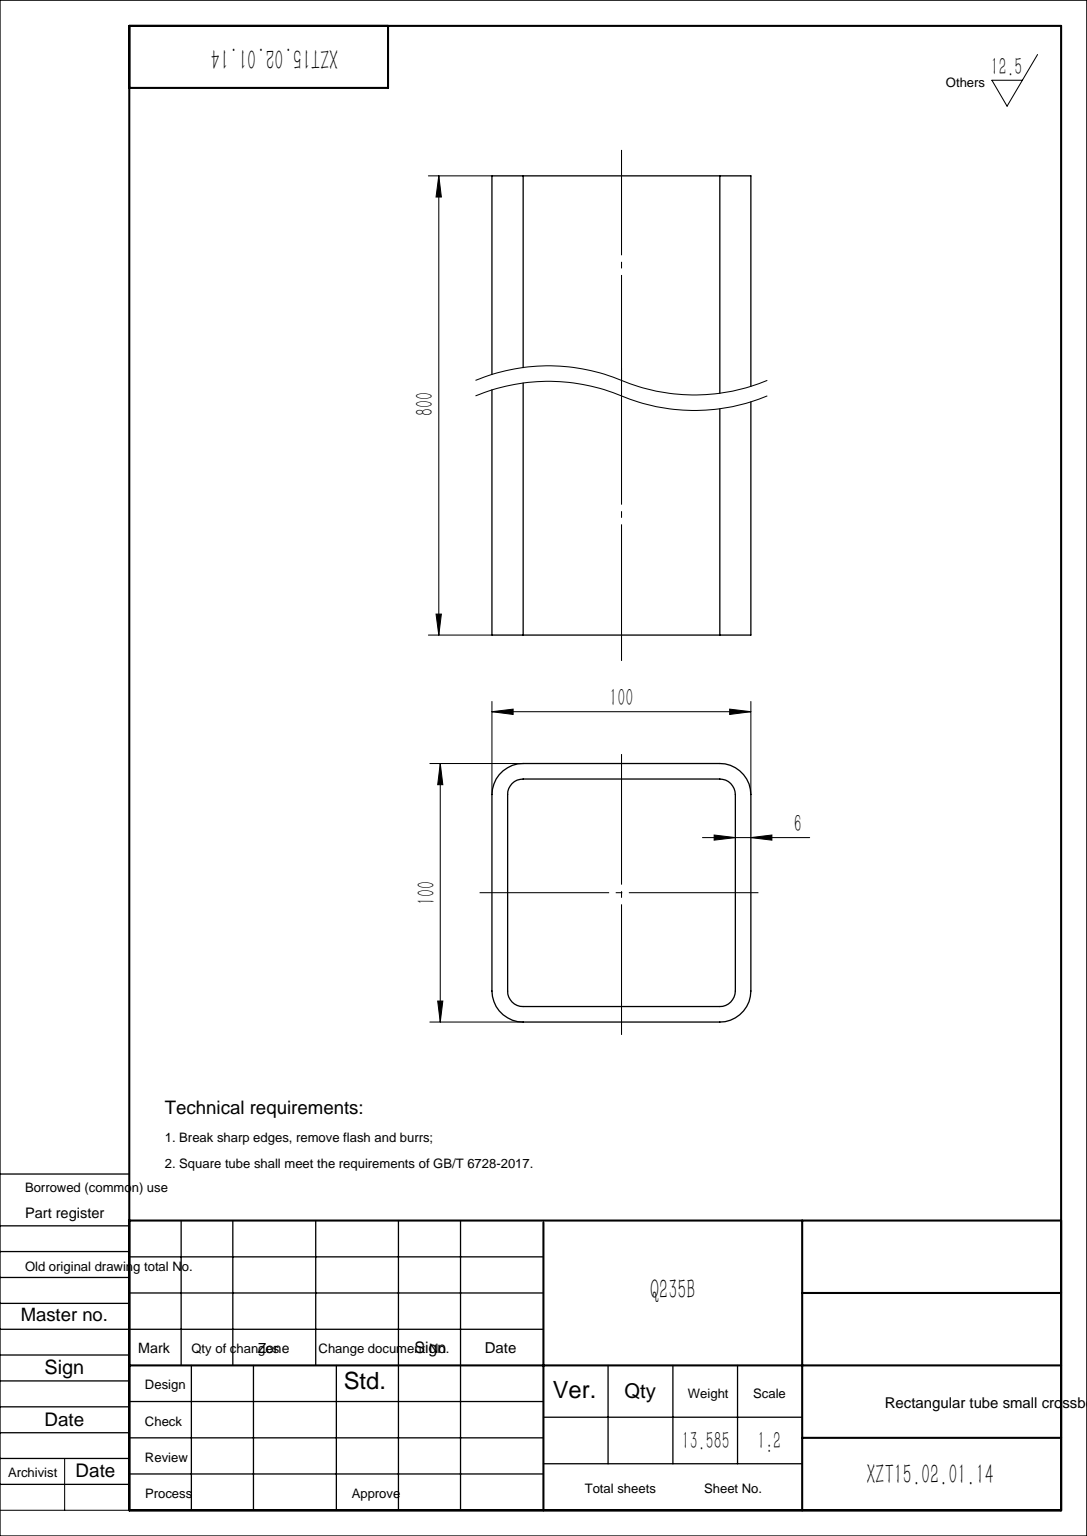
SolidWorks part; units mm, degrees
material "Q235B"
ref_plane "Front Plane" through (0, 0, 0) normal (0, 0, 1) x (1, 0, 0)
ref_plane "Top Plane" through (0, 0, 0) normal (0, 1, 0) x (1, 0, 0)
ref_plane "Right Plane" through (0, 0, 0) normal (1, 0, 0) x (0, 0, -1)
sketch "Sketch1" plane through (0, 0, 0) normal (0, 0, 1) x (1, 0, 0)
  line L0 (0, 0) -> (0, 800)
  dimension "D1" = 800
other "GB/T 6728-2002 square hollow section 100×100×6(1)"
ref_plane "Plane1" through (0, 0, 0) normal (0, 1, 0) x (-1, 0, 0)
sketch "Sketch11" plane through (0, 0, 0) normal (0, 1, 0) x (-1, 0, 0)
  line L0 (-38, -44) -> (38, -44)
  line L1 (-44, -38) -> (-44, 38)
  line L2 (38, 44) -> (-38, 44)
  line L3 (44, 38) -> (44, -38)
  line L4 (-38, -50) -> (38, -50)
  line L5 (-50, -38) -> (-50, 38)
  line L6 (38, 50) -> (-38, 50)
  line L7 (50, 38) -> (50, -38)
  arc A0 (50, 38) -> (38, 50) centre (38, 38) ccw
  arc A1 (38, -50) -> (50, -38) centre (38, -38) ccw
  arc A2 (-50, -38) -> (-38, -50) centre (-38, -38) ccw
  arc A3 (-38, 50) -> (-50, 38) centre (-38, 38) ccw
  arc A4 (-38, 44) -> (-44, 38) centre (-38, 38) ccw
  arc A5 (44, 38) -> (38, 44) centre (38, 38) ccw
  arc A6 (38, -44) -> (44, -38) centre (38, -38) ccw
  arc A7 (-44, -38) -> (-38, -44) centre (-38, -38) ccw
  point P0 (-50, 0)
  point P1 (50, 0)
  point P2 (0, 50)
  point P3 (0, -50)
  point P4 (0, 0)
  point P5 (-50, -50)
  point P6 (50, -50)
  point P7 (50, 50)
  point P8 (-50, 50)
  point P33 (0, 0)
  dimension "D1" = 12
  dimension "Thickness" = 6
  dimension "V_leg" = 100
